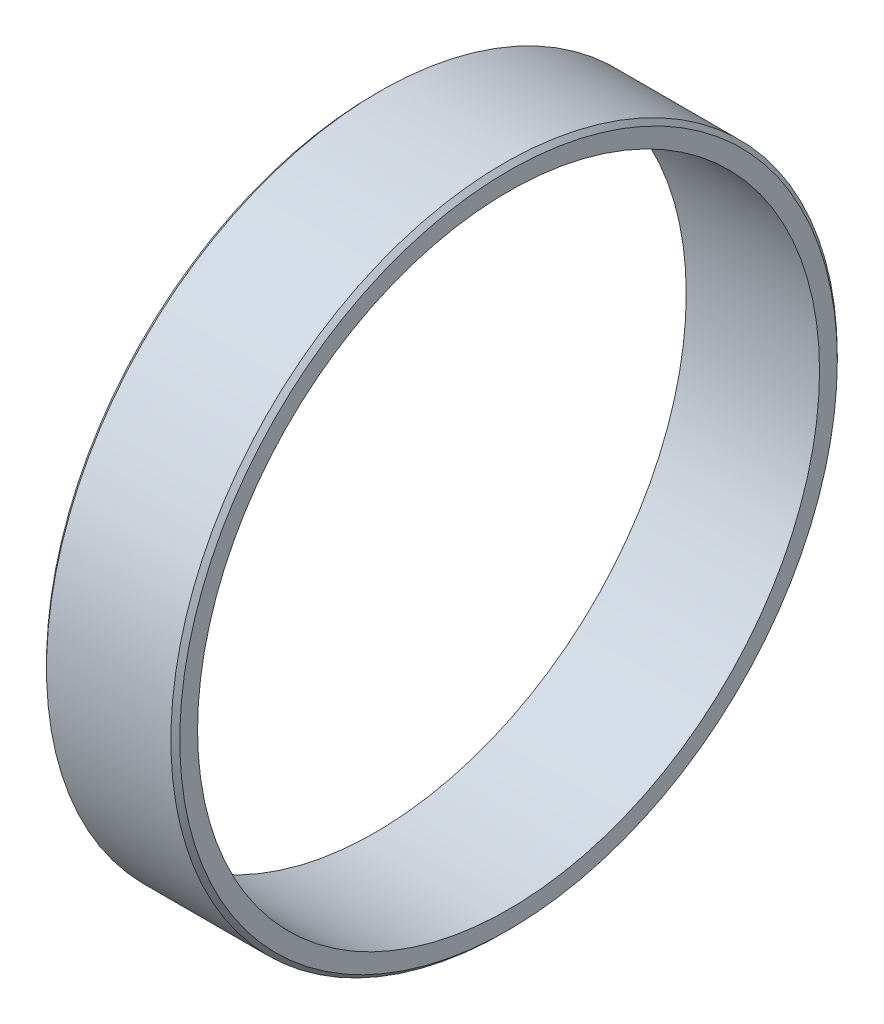
from build123d import *

# Parameters (mm, degrees)
SKETCH2_R           = 37.5
SKETCH2_R_2         = 35
BOSS_EXTRUDE1_DEPTH = 15
CHAMFER1_SIZE       = 0.5


with BuildPart() as part:
    # Sketch2 → Boss-Extrude1 (new body)
    with BuildSketch(Plane(origin=(0, 0, 0), x_dir=(0, 0, -1), z_dir=(1, 0, 0))):
        Circle(SKETCH2_R)
        Circle(SKETCH2_R_2, mode=Mode.SUBTRACT)
    extrude(amount=-BOSS_EXTRUDE1_DEPTH)

    # Chamfer1
    chamfer1_edges = [part.edges().sort_by_distance(p)[0] for p in [
        (0, 0, 37.5),
        (-15, 0, 37.5),
    ]]
    chamfer(chamfer1_edges, length=CHAMFER1_SIZE)


solid = part.part
